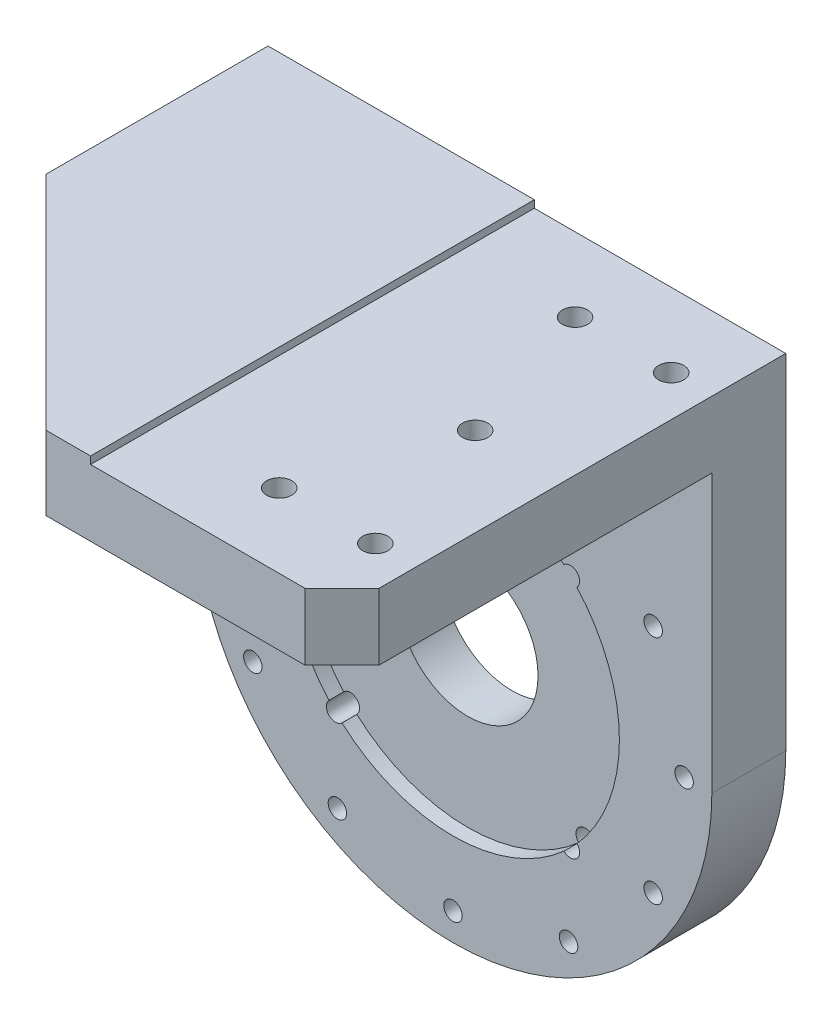
SolidWorks part; units mm, degrees
material "6061Al"
ref_plane "前视基准面" through (0, 0, 0) normal (0, 0, 1) x (1, 0, 0)
ref_plane "上视基准面" through (0, 0, 0) normal (0, 1, 0) x (1, 0, 0)
ref_plane "右视基准面" through (0, 0, 0) normal (1, 0, 0) x (0, 0, -1)
sketch "草图1" plane through (0, 0, 0) normal (0, 0, 1) x (1, 0, 0)
  line L0 (-70, 0) -> (-70, 75)
  line L1 (-70, 75) -> (70, 75)
  line L2 (70, 75) -> (70, 0)
  arc A0 (-70, 0) -> (70, 0) centre (0, 0) ccw
  dimension "D1" = 140
  dimension "D2" = 75
extrude "凸台-拉伸1" add sketch "草图1" along normal blind 20
sketch "草图2" plane through (0, 0, 20) normal (0, 0, 1) x (1, 0, 0)
  circle A0 centre (0, 0) radius 45
  dimension "D1" = 90
extrude "切除-拉伸1" cut sketch "草图2" against normal blind 4
sketch "草图3" plane through (0, 0, 16) normal (0, 0, 1) x (1, 0, 0)
  circle A0 centre (0, 0) radius 19
  dimension "D1" = 38
extrude "切除-拉伸2" cut sketch "草图3" against normal through all
sketch "草图4" plane through (0, 0, 0) normal (0, 0, -1) x (-1, 0, 0)
  circle A0 centre (0, 0) radius 35
  dimension "D1" = 70
extrude "切除-拉伸3" cut sketch "草图4" against normal blind 4
hole_wizard "M6 螺纹孔1" positions "草图5" profile "草图6" tap size "M6" standard "ISO" end condition through all
sketch "草图5" plane through (0, 0, 20) normal (0, 0, 1) x (1, 0, 0)
  line L0 (0, 0) -> (0, 62.5) construction
  point P0 (0, 62.5)
  point P9 (31.25, 54.1266)
  point P10 (54.1266, 31.25)
  point P11 (62.5, 0)
  point P12 (54.1266, -31.25)
  point P13 (31.25, -54.1266)
  point P14 (0, -62.5)
  point P15 (-31.25, -54.1266)
  point P16 (-54.1266, -31.25)
  point P17 (-62.5, 0)
  point P18 (-54.1266, 31.25)
  point P19 (-31.25, 54.1266)
  dimension "D3" = 62.5
  dimension "D2" = 12
sketch "草图6" plane through (0, 62.5, 20) normal (1, 0, 0) x (0, -1, 0)
  line L0 (0, 0) -> (0, 20)
  line L1 (0, 20) -> (2.5, 20)
  line L2 (2.5, 20) -> (2.5, 0)
  line L5 (2.5, 0) -> (0, 0)
  line L11 (0, -6.35) -> (0, 107.95) construction
  dimension "通孔螺纹孔钻头直径" = 5
  dimension "通孔螺纹孔钻头深度" = 20
cosmetic thread "孔螺蚊线1" parameters "D2"=6
cosmetic thread "孔螺蚊线2" parameters "D2"=6
cosmetic thread "孔螺蚊线3" parameters "D2"=6
cosmetic thread "孔螺蚊线4" parameters "D2"=6
cosmetic thread "孔螺蚊线5" parameters "D2"=6
cosmetic thread "孔螺蚊线6" parameters "D2"=6
cosmetic thread "孔螺蚊线7" parameters "D2"=6
cosmetic thread "孔螺蚊线8" parameters "D2"=6
cosmetic thread "孔螺蚊线9" parameters "D2"=6
cosmetic thread "孔螺蚊线10" parameters "D2"=6
cosmetic thread "孔螺蚊线11" parameters "D2"=6
cosmetic thread "孔螺蚊线12" parameters "D2"=6
hole_wizard "M6 螺纹孔2" positions "草图7" profile "草图8" tap size "M6" standard "ISO" end condition through all
sketch "草图7" plane through (0, 0, 20) normal (0, 0, 1) x (1, 0, 0)
  line L1 (-31.75, -31.75) -> (31.75, -31.75)
  line L2 (-31.75, -31.75) -> (-31.75, 31.75)
  line L3 (-31.75, 31.75) -> (31.75, 31.75)
  line L4 (31.75, -31.75) -> (31.75, 31.75)
  line L5 (-31.75, -31.75) -> (31.75, 31.75) construction
  line L6 (-31.75, 31.75) -> (31.75, -31.75) construction
  point P3 (0, 0)
  point P4 (31.75, 31.75)
  point P33 (-31.75, -31.75)
  point P34 (-31.75, 31.75)
  point P35 (31.75, -31.75)
  dimension "D1" = 63.5
sketch "草图8" plane through (0, 0, 20) normal (1, 0, 0) x (0, -1, 0)
  line L0 (0, 0) -> (0, 20)
  line L1 (0, 20) -> (2.5, 20)
  line L2 (2.5, 20) -> (2.5, 0)
  line L5 (2.5, 0) -> (0, 0)
  line L11 (0, -6.35) -> (0, 107.95) construction
  dimension "通孔螺纹孔钻头直径" = 5
  dimension "通孔螺纹孔钻头深度" = 20
cosmetic thread "孔螺蚊线13" parameters "D2"=6
cosmetic thread "孔螺蚊线14" parameters "D2"=6
cosmetic thread "孔螺蚊线15" parameters "D2"=6
cosmetic thread "孔螺蚊线16" parameters "D2"=6
sketch "草图15" plane through (0, 75, 0) normal (0, 1, 0) x (1, 0, 0)
  line L0 (70, -20) -> (70, 0) construction
  line L1 (-70, 0) -> (70, 0)
  line L2 (-70, 0) -> (-70, -120)
  line L3 (-70, -120) -> (70, -120)
  line L4 (70, 0) -> (70, -120)
  dimension "D1" = 120
extrude "凸台-拉伸2" add sketch "草图15" along normal blind 20
sketch "草图20" plane through (0, 95, 0) normal (0, 1, 0) x (1, 0, 0)
  line L0 (-70, -120) -> (70, -120) construction
  line L1 (2, 0) -> (70, 0)
  line L2 (2, 0) -> (2, -120)
  line L3 (2, -120) -> (70, -120)
  line L4 (70, 0) -> (70, -120)
  dimension "D1" = 68
extrude "切除-拉伸4" cut sketch "草图20" against normal blind 2
chamfer "倒角1" distance 10 angle 45 1 edges at (70, 84, 120)
chamfer "倒角2" distance 60 angle 45 1 edges at (-70, 85, 120)
hole_wizard "M8 螺纹孔1" positions "草图21" profile "草图22" tap size "M8" standard "ISO" end condition up to next
sketch "草图21" plane through (0, 95, 0) normal (0, 1, 0) x (1, 0, 0)
  point P0 (33, -20)
  point P3 (59, -20)
  point P6 (46, -60)
  point P9 (33, -100)
  point P12 (59, -100)
sketch "草图22" plane through (33, 95, 20) normal (1, 0, 0) x (0, 0, 1)
  line L0 (0, 0) -> (0, 20)
  line L1 (0, 20) -> (3.4, 20)
  line L2 (3.4, 20) -> (3.4, 0)
  line L5 (3.4, 0) -> (0, 0)
  line L11 (0, -6.35) -> (0, 107.95) construction
  dimension "通孔螺纹孔钻头直径" = 6.8
  dimension "通孔螺纹孔钻头深度" = 20
cosmetic thread "孔螺蚊线17" parameters "D2"=8
cosmetic thread "孔螺蚊线18" parameters "D2"=8
cosmetic thread "孔螺蚊线19" parameters "D2"=8
cosmetic thread "孔螺蚊线20" parameters "D2"=8
cosmetic thread "孔螺蚊线21" parameters "D2"=8
